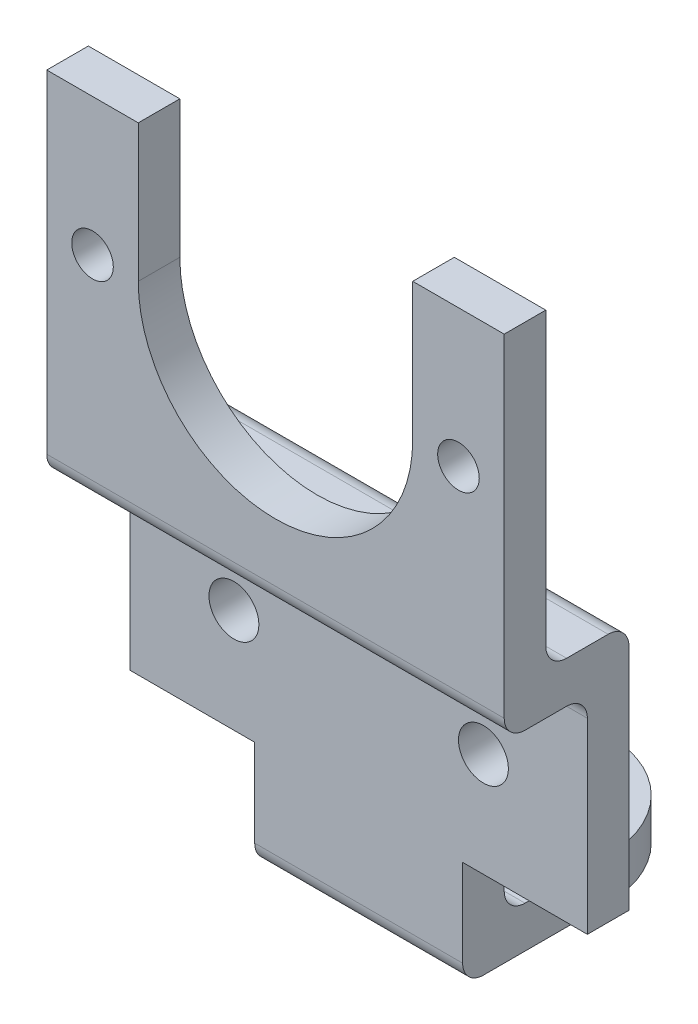
from build123d import *

# Parameters (mm, degrees)
SKETCH_1_R           = 6
EXTRUDE_1_DEPTH      = 10
SKETCH_2_W           = 50
SKETCH_2_H           = 10
EXTRUDE_2_DEPTH      = 60
SKETCH_3_R           = 12.5
CUT_EXTRUDE_1_DEPTH  = 10
FILLET_1_R           = 5
EXTRUDE_3_DEPTH      = 10
EXTRUDE_3_DEPTH_BACK = 10
SKETCH_5_W           = 110
SKETCH_5_H           = 10
SKETCH_6_R           = 5
EXTRUDE_4_DEPTH      = 10
FILLET_2_R           = 5


with BuildPart() as part:
    # 草图1 → 凸台-拉伸1 (new body)
    with BuildSketch(Plane.XY):
        Polygon((-55, 50), (55, 50), (55, 0), (50, 0), (25, 0), (25, -16), (-25, -16), (-25, 0), (-55, 0), align=None)
        with Locations((-30, 25)):
            Circle(SKETCH_1_R, mode=Mode.SUBTRACT)
        with Locations((30, 25)):
            Circle(SKETCH_1_R, mode=Mode.SUBTRACT)
    extrude(amount=EXTRUDE_1_DEPTH)

    # 草图2 → 凸台-拉伸2 (add)
    with BuildSketch(Plane.XY.offset(10)):
        with Locations((0, -21)):
            Rectangle(SKETCH_2_W, SKETCH_2_H)
    extrude(amount=-EXTRUDE_2_DEPTH)

    # 草图3 → 切除-拉伸1 (cut)
    with BuildSketch(Plane(origin=(0, -16, 0), x_dir=(1, 0, 0), z_dir=(0, 1, 0))):
        with Locations(Location((0, 25, 0), (0, 0, 180))):
            Circle(SKETCH_3_R)
        with BuildLine():
            Line((-25, 25), (-25, 57.057636161))
            Line((-25, 57.057636161), (25, 57.057636161))
            Line((25, 57.057636161), (25, 25))
            ThreePointArc((25, 25), (0, 50), (-25, 25))
        make_face()
    extrude(amount=-CUT_EXTRUDE_1_DEPTH, mode=Mode.SUBTRACT)

    # 圆角1
    fillet_1_edges = [part.edges().sort_by_distance(p)[0] for p in [
        (0, -16, 0),
        (0, -26, 10),
    ]]
    fillet(fillet_1_edges, radius=FILLET_1_R)

    # 草图5 → 凸台-拉伸3 (add, two sides: drawn at the far end of the back side and taken through both)
    with BuildSketch(Plane.XY.offset(10).offset(-EXTRUDE_3_DEPTH_BACK)):
        with Locations((0, 55)):
            Rectangle(SKETCH_5_W, SKETCH_5_H)
    extrude(amount=EXTRUDE_3_DEPTH + EXTRUDE_3_DEPTH_BACK)

    # 草图6 → 凸台-拉伸4 (add)
    with BuildSketch(Plane.XY.offset(20)):
        with BuildLine():
            Line((-55, 60), (-55, 135))
            Line((-55, 135), (-33, 135))
            Line((-33, 135), (-33, 102))
            ThreePointArc((-33, 102), (0, 69), (33, 102))
            Line((33, 102), (33, 135))
            Line((33, 135), (55, 135))
            Line((55, 135), (55, 60))
            Line((55, 60), (55, 50))
            Line((55, 50), (-55, 50))
            Line((-55, 50), (-55, 60))
        make_face()
        with Locations((44, 102)):
            Circle(SKETCH_6_R, mode=Mode.SUBTRACT)
        with Locations((-44, 102)):
            Circle(SKETCH_6_R, mode=Mode.SUBTRACT)
    extrude(amount=EXTRUDE_4_DEPTH)

    # 圆角2
    fillet_2_edges = [part.edges().sort_by_distance(p)[0] for p in [
        (0, 50, 10),
        (0, 50, 30),
        (0, 60, 20),
        (0, 60, 0),
    ]]
    fillet(fillet_2_edges, radius=FILLET_2_R)


solid = part.part
